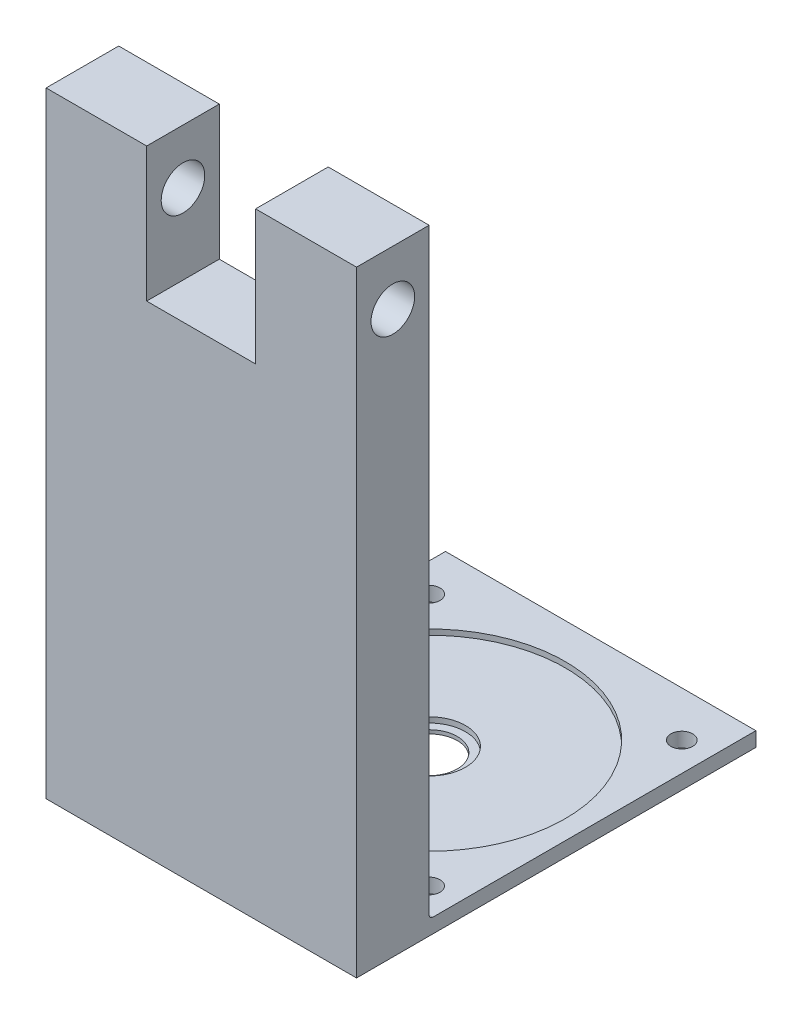
SolidWorks part; units mm, degrees
material "铝合金板 LF5"
ref_plane "前视基准面" through (0, 0, 0) normal (0, 0, 1) x (1, 0, 0)
ref_plane "上视基准面" through (0, 0, 0) normal (0, 1, 0) x (1, 0, 0)
ref_plane "右视基准面" through (0, 0, 0) normal (1, 0, 0) x (0, 0, -1)
sketch "草图1" plane through (0, 0, 0) normal (0, 0, 1) x (1, 0, 0)
  line L2 (-42.75, -59) -> (-42.75, 59)
  line L4 (42.75, -59) -> (42.75, 59)
  line L5 (-42.75, -59) -> (42.75, 59) construction
  line L6 (-42.75, 59) -> (42.75, -59) construction
  line L9 (-42.75, -59) -> (42.75, -59)
  line L10 (-42.75, 59) -> (-42.75, 129)
  line L11 (-42.75, 129) -> (42.75, 129)
  line L12 (42.75, 129) -> (42.75, 59)
  point P0 (0, 0)
  dimension "D1" = 118
  dimension "D2" = 85.5
  dimension "D3" = 70
extrude "凸台-拉伸1" add sketch "草图1" along normal blind 20
sketch "草图2" plane through (0, 0, 20) normal (0, 0, 1) x (1, 0, 0)
  line L8 (-15.052, 92) -> (-15.052, 129)
  line L9 (42.75, 129) -> (-42.75, 129) construction
  line L10 (-15.052, 129) -> (14.948, 129)
  line L11 (14.948, 129) -> (14.948, 92)
  line L12 (-15.052, 92) -> (14.948, 92)
  point P0 (-0.052, 40.5)
  dimension "D3" = 37
extrude "切除-拉伸1" cut sketch "草图2" against normal blind 20
sketch "草图3" plane through (-42.75, 0, 0) normal (-1, 0, 0) x (0, 0, 1)
  line L0 (10, 129) -> (10, 92.3514) construction
  line L2 (20, 129) -> (0, 129) construction
  circle A0 centre (10, 114) radius 6
  dimension "D1" = 12
  dimension "D2" = 15
extrude "切除-拉伸2" cut sketch "草图3" against normal through all both and the other way through all
sketch "草图4" plane through (0, 0, 20) normal (0, 0, 1) x (1, 0, 0)
  line L0 (42.75, -59) -> (42.75, 129) construction
  line L1 (-42.75, -59) -> (42.75, -59)
  line L2 (-42.75, -59) -> (-42.75, -49)
  line L3 (-42.75, -49) -> (42.75, -49)
  line L4 (42.75, -59) -> (42.75, -49)
  dimension "D1" = 10
extrude "切除-拉伸3" cut sketch "草图4" against normal through all both and the other way through all
sketch "草图5" plane through (0, -49, 0) normal (0, -1, 0) x (1, 0, 0)
  line L4 (42.75, 20) -> (-42.75, 20)
  line L5 (-42.75, 20) -> (-42.75, 0)
  line L6 (-42.75, 0) -> (42.75, 0)
  line L7 (42.75, 0) -> (42.75, 20)
  line L8 (42.75, 20) -> (-42.75, 20)
  line L9 (-42.75, 20) -> (-42.75, 0)
  line L10 (-42.75, 0) -> (42.75, 0)
  line L11 (42.75, 0) -> (42.75, 20)
  dimension "D1" = 0
extrude "切除-拉伸4" cut sketch "草图5" against normal blind 8.43
sketch "草图6" plane through (0, 0, 20) normal (0, 0, 1) x (1, 0, 0)
  line L0 (42.75, -40.57) -> (42.75, 129) construction
  line L1 (-42.75, -40.57) -> (42.75, -40.57)
  line L2 (-42.75, -40.57) -> (-42.75, -36.57)
  line L3 (-42.75, -36.57) -> (42.75, -36.57)
  line L4 (42.75, -40.57) -> (42.75, -36.57)
  dimension "D1" = 4
extrude "凸台-拉伸2" add sketch "草图6" against normal blind 90 from surface at -20 starting at face at (-0.026, 77.3575, 0)
sketch "草图8" plane through (0, -36.57, 0) normal (0, 1, 0) x (1, 0, 0)
  circle A0 centre (-34.8, 77.55) radius 3
  circle A1 centre (34.8, 77.55) radius 3
  circle A2 centre (-34.8, 7.95) radius 3
  circle A3 centre (34.8, 7.95) radius 3
  dimension "D1" = 6
extrude "切除-拉伸6" cut sketch "草图8" against normal blind 90
fillet "圆角1" radius 1 1 edges at (0, -36.57, 0)
sketch "草图9" plane through (0, -36.57, 0) normal (0, 1, 0) x (1, 0, 0)
  line L0 (-34.8, 77.55) -> (34.8, 7.95) construction
  line L1 (34.8, 77.55) -> (-34.8, 7.95) construction
  circle A0 centre (0, 42.75) radius 37.5
  dimension "D1" = 75
extrude "切除-拉伸7" cut sketch "草图9" against normal blind 1.5
sketch "草图10" plane through (0, -38.07, 0) normal (0, 1, 0) x (1, 0, 0)
  circle A0 centre (0, 42.75) radius 7.75
  dimension "D1" = 15.5
extrude "切除-拉伸8" cut sketch "草图10" against normal through all both and the other way through all
sketch "草图11" plane through (0, -38.07, 0) normal (0, 1, 0) x (1, 0, 0)
  circle A0 centre (0, 42.75) radius 10
  dimension "D1" = 20
extrude "切除-拉伸9" cut sketch "草图11" against normal blind 1.5
